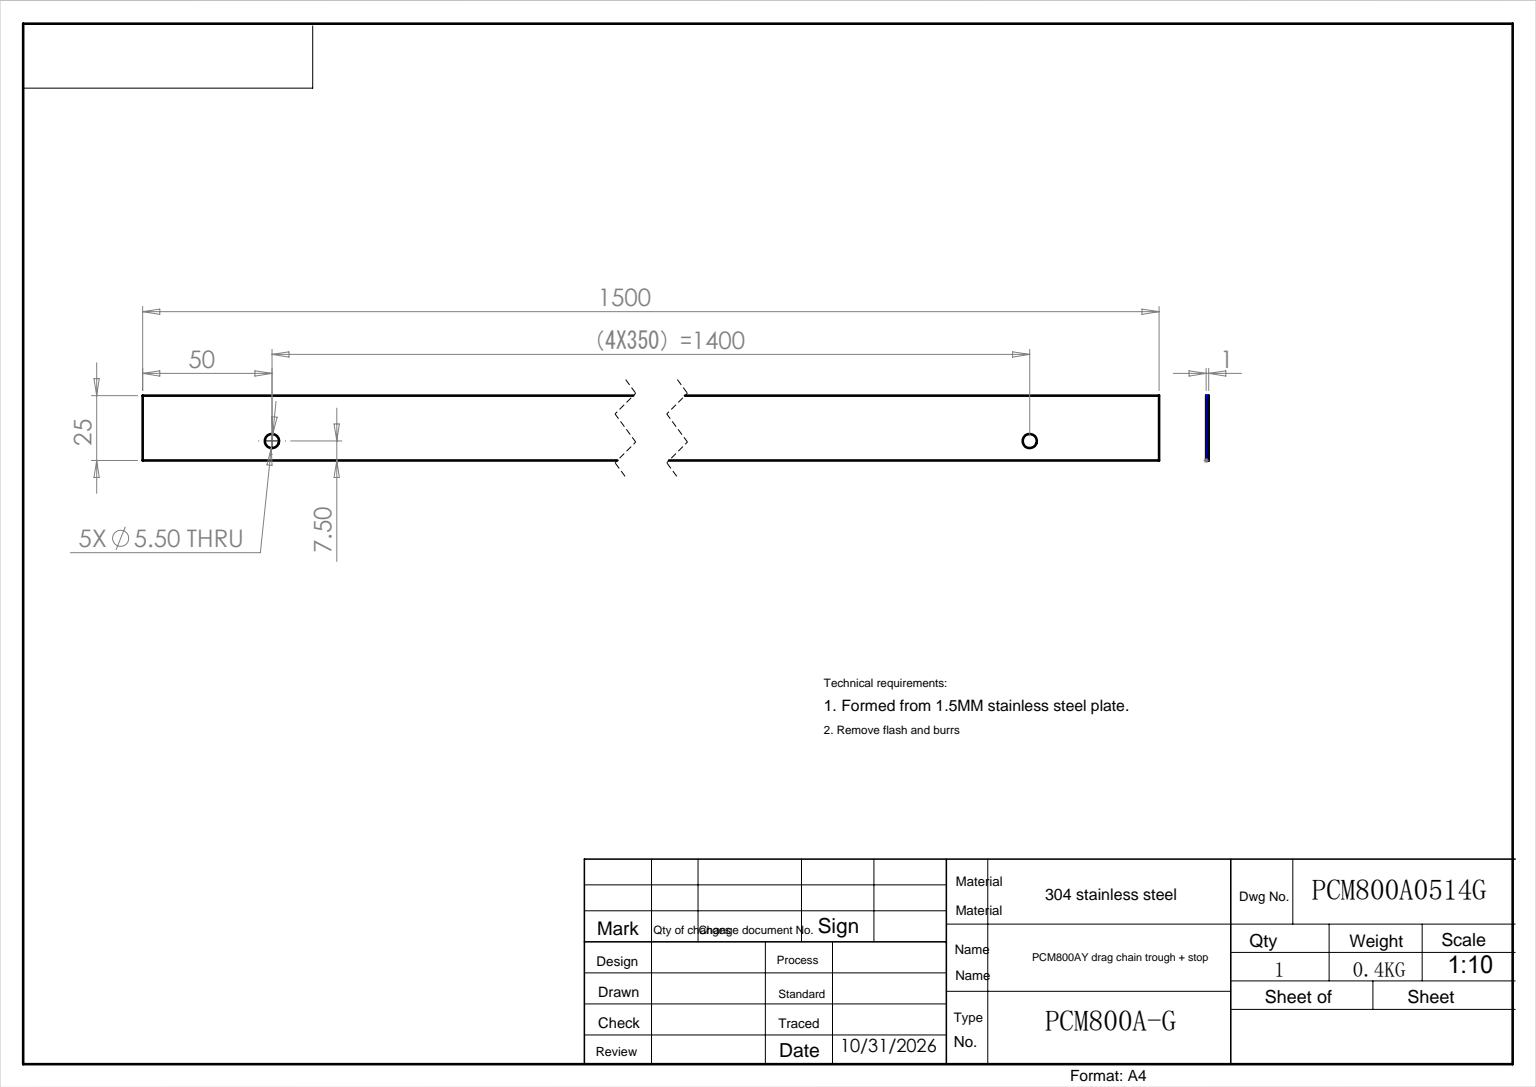
SolidWorks part; units mm, degrees
ref_plane "前视基准面" through (0, 0, 0) normal (0, 0, 1) x (1, 0, 0)
ref_plane "上视基准面" through (0, 0, 0) normal (0, 1, 0) x (1, 0, 0)
ref_plane "右视基准面" through (0, 0, 0) normal (1, 0, 0) x (0, 0, -1)
sketch "草图1" plane through (0, 0, 0) normal (0, 0, 1) x (1, 0, 0)
  line L1 (0, 0) -> (1500, 0)
  line L2 (0, 0) -> (0, 25)
  line L3 (0, 25) -> (1500, 25)
  line L4 (1500, 0) -> (1500, 25)
  dimension "D1" = 1500
  dimension "D2" = 25
extrude "凸台-拉伸1" add sketch "草图1" along normal blind 1
sketch "草图2" plane through (0, 0, 1) normal (0, 0, 1) x (1, 0, 0)
  line L0 (-23.8725, 7.5) -> (1483.5623, 7.5) construction
  line L1 (0, 0) -> (1500, 0) construction
  line L2 (0, 25) -> (0, 0) construction
  circle A0 centre (50, 7.5) radius 2.75
  circle A1 centre (400, 7.5) radius 2.75
  circle A2 centre (750, 7.5) radius 2.75
  circle A3 centre (1100, 7.5) radius 2.75
  circle A4 centre (1450, 7.5) radius 2.75
  dimension "D2" = 5.5
  dimension "D3" = 50
  dimension "D1" = 7.5
extrude "切除-拉伸1" cut sketch "草图2" against normal blind 10
